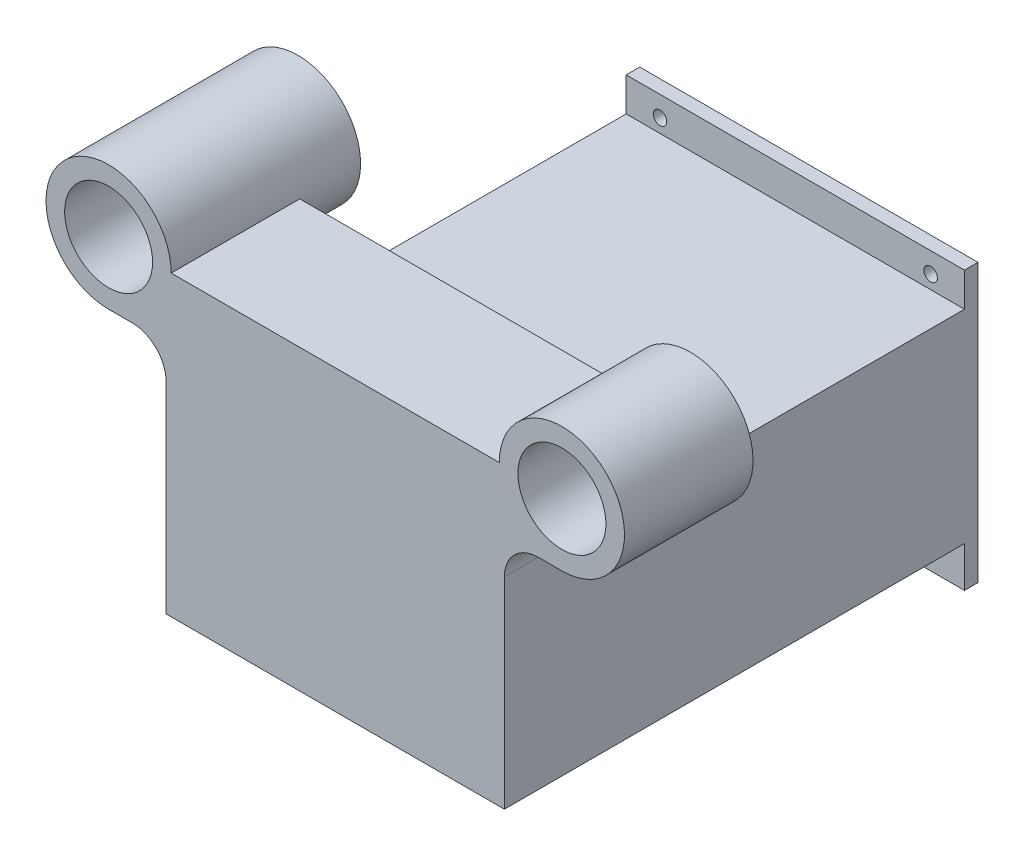
SolidWorks part; units mm, degrees
ref_plane "前视基准面" through (0, 0, 0) normal (0, 0, 1) x (1, 0, 0)
ref_plane "上视基准面" through (0, 0, 0) normal (0, 1, 0) x (1, 0, 0)
ref_plane "右视基准面" through (0, 0, 0) normal (1, 0, 0) x (0, 0, -1)
other "Configuration Table"
sketch "草图2" plane through (0, 0, 0) normal (0, 0, 1) x (1, 0, 0)
  line L0 (-77.659, 0) -> (85.7057, 0) construction
  line L1 (0, 83.4614) -> (0, -111.0062) construction
  line L2 (-48.5, 0) -> (48.5, 0)
  line L3 (-103.5759, -88) -> (110.5941, -88) construction
  line L4 (50, -88) -> (-50, -88)
  line L5 (-50, -88) -> (-50, -28.5)
  line L6 (-67, -18.5) -> (-60, -18.5)
  line L7 (50, -88) -> (50, -28.5)
  line L8 (67, -18.5) -> (60, -18.5)
  circle A0 centre (-67, 0) radius 13
  circle A1 centre (67, 0) radius 13
  arc A2 (-48.5, 0) -> (-67, -18.5) centre (-67, 0) ccw
  arc A3 (-50, -28.5) -> (-60, -18.5) centre (-60, -28.5) ccw
  arc A4 (50, -28.5) -> (60, -18.5) centre (60, -28.5) cw
  arc A5 (48.5, 0) -> (67, -18.5) centre (67, 0) cw
  point P22 (0, 0)
  point P23 (0, -88)
  dimension "D1" = 134
  dimension "D6" = 26
  dimension "D3" = 50
extrude "凸台-拉伸1" add sketch "草图2" along normal blind 38
sketch "草图23" plane through (0, 0, 0) normal (0, 0, -1) x (-1, 0, 0)
  line L0 (-50, -88) -> (-50, -28)
  line L1 (-50, -28) -> (50, -28)
  line L2 (50, -28) -> (50, -88)
  line L3 (50, -88) -> (-50, -88)
  line L4 (-59.7699, -78) -> (68.4113, -78) construction
  line L9 (-46, -78) -> (46, -78)
  line L10 (0, -29.7211) -> (0, -88) construction
  line L11 (-46, -78) -> (-46, -36)
  line L12 (-46, -36) -> (46, -36)
  line L13 (46, -78) -> (46, -36)
  point P10 (0, -78)
  point P11 (0, -36)
  point P16 (0, -78)
  point P17 (0, -36)
  dimension "D1" = 60
  dimension "D2" = 10
  dimension "D3" = 4
  dimension "D4" = 42
  dimension "D5" = 92
extrude "凸台-拉伸7" add sketch "草图23" along normal blind 102
ref_plane "基准面8" through (0, -88, 0) normal (0, -1, 0) x (-1, 0, 0)
sketch "草图25" plane through (0, -88, 0) normal (0, -1, 0) x (-1, 0, 0)
  line L0 (0, 41.9664) -> (0, -57.2775) construction
  line L1 (50, -38) -> (-50, -38) construction
  circle A0 centre (0, 14) radius 7
  dimension "D1" = 14
  dimension "D2" = 52
extrude "切除-拉伸4" cut sketch "草图25" against normal blind 50
ref_plane "基准面9" through (0, 0, 0) normal (0, 0, -1) x (-1, 0, 0)
sketch "草图26" plane through (0, 0, 0) normal (0, 0, -1) x (-1, 0, 0)
  circle A0 centre (67, 0) radius 13
  circle A1 centre (67, 0) radius 18.5
extrude "凸台-拉伸8" add sketch "草图26" along normal blind 18
sketch "草图28" plane through (0, 0, 0) normal (0, 0, -1) x (-1, 0, 0)
  line L0 (-46, -36) -> (-46, -78)
  line L1 (-46, -78) -> (46, -78)
  line L2 (46, -78) -> (46, -36)
  line L3 (46, -36) -> (-46, -36)
extrude "切除-拉伸5" cut sketch "草图28" against normal blind 30
ref_plane "基准面10" through (0, 0, -14) normal (0, 0, 1) x (1, 0, 0)
ref_plane "基准面11" through (0, -36, 0) normal (0, -1, 0) x (-1, 0, 0)
sketch "草图29" plane through (0, -36, 0) normal (0, -1, 0) x (-1, 0, 0)
  line L0 (0, 43.1114) -> (0, -38) construction
  line L1 (50, -38) -> (-50, -38) construction
  line L2 (-52.8549, -30.0159) -> (57.6218, -30.0159) construction
  line L3 (-46, -19.9504) -> (-46, -40.813) construction
  line L4 (-50, -38) -> (-50, 102) construction
  line L5 (-46, -30.0159) -> (46, -30.0159)
  line L6 (-46, -30.0159) -> (-46, 36.9841)
  line L7 (-46, 36.9841) -> (46, 36.9841)
  line L8 (46, -30.0159) -> (46, 36.9841)
  point P15 (0, -30.0159)
  point P16 (0, 36.9841)
  dimension "D1" = 7.9841
  dimension "D2" = 4
extrude "凸台-拉伸9" add sketch "草图29" along normal blind 4
sketch "草图30" plane through (0, 0, -14) normal (0, 0, 1) x (1, 0, 0)
  line L0 (0, 34.4581) -> (0, -88) construction
  line L1 (-50, -88) -> (50, -88) construction
  line L2 (0, -88) -> (-8, -88)
  line L3 (-8, -88) -> (-8, -85.4)
  line L4 (-8, -85.4) -> (-12, -85.4)
  line L5 (-12, -85.4) -> (-12, -84.256)
  line L6 (-12, -84.256) -> (-14, -84.256)
  line L7 (-14, -84.256) -> (-14, -36.1145)
  line L8 (-14, -36.1145) -> (-7.5, -36.1145)
  line L9 (-7.5, -36.1145) -> (-7.5, -35)
  line L10 (-7.5, -35) -> (-7, -35)
  line L11 (-7, -35) -> (-7, -31.9)
  line L12 (-7, -31.9) -> (0, -31.9)
  line L13 (0, -88) -> (0, -31.9)
revolve "切除-旋转3" cut sketch "草图30" angle 360 about L13
ref_plane "基准面12" through (0, 0, -59.8) normal (0, 0, 1) x (1, 0, 0)
sketch "草图31" plane through (0, 0, -59.8) normal (0, 0, 1) x (1, 0, 0)
  line L0 (0, 18.5373) -> (0, -105.0668) construction
  line L1 (-81.3892, -84.7) -> (88.7308, -84.7) construction
  line L2 (-55, -88) -> (55, -88) construction
  line L3 (0, -84.7) -> (-6.7, -84.7)
  line L4 (-6.7, -84.7) -> (-6.7, -82.7)
  line L5 (-6.7, -82.7) -> (-7.5, -82.7)
  line L6 (-7.5, -82.7) -> (-7.5, -30.816)
  line L7 (-7.5, -30.816) -> (-6.7, -30.816)
  line L8 (-6.7, -30.816) -> (-6.7, -28.816)
  line L9 (-6.7, -28.816) -> (0, -28.816)
  line L10 (0, -84.7) -> (0, -28.816)
  dimension "D1" = 3.3
revolve "切除-旋转4" cut sketch "草图31" angle 360 about L10
ref_plane "基准面13" through (0, 0, -102) normal (0, 0, -1) x (-1, 0, 0)
sketch "草图32" plane through (0, 0, -102) normal (0, 0, -1) x (-1, 0, 0)
  line L0 (-50, -28) -> (-50, -18)
  line L1 (-50, -18) -> (50, -18)
  line L2 (50, -18) -> (50, -28)
  line L3 (-50, -28) -> (50, -28)
  line L4 (-50, -88) -> (-50, -100)
  line L5 (-55, -88) -> (55, -88) construction
  line L6 (-50, -100) -> (50, -100)
  line L7 (50, -100) -> (50, -88)
  line L8 (50, -88) -> (50, -28) construction
  line L9 (-50, -88) -> (50, -88)
extrude "凸台-拉伸10" add sketch "草图32" against normal blind 4
sketch "草图33" plane through (0, 0, -102) normal (0, 0, -1) x (-1, 0, 0)
  line L0 (-40, -79.8879) -> (-40, -108.2271) construction
  line L1 (-50, -18) -> (-50, -100) construction
  line L2 (-52.0127, -94) -> (-28.6632, -94) construction
  line L3 (-50, -100) -> (50, -100) construction
  line L4 (-40, -15.2314) -> (-40, -27.9512) construction
  line L5 (-51.316, -24) -> (-37.5442, -24) construction
  line L6 (50, -18) -> (-50, -18) construction
  line L7 (0, 17.9843) -> (0, -116.3235) construction
  circle A0 centre (-40, -94.0575) radius 2
  circle A1 centre (-40, -24) radius 2
  circle A2 centre (40, -94.0575) radius 2
  circle A3 centre (40, -24) radius 2
  dimension "D3" = 4
  dimension "D1" = 10
  dimension "D2" = 6
  dimension "D4" = 10
  dimension "D5" = 6
extrude "切除-拉伸6" cut sketch "草图33" against normal blind 4
